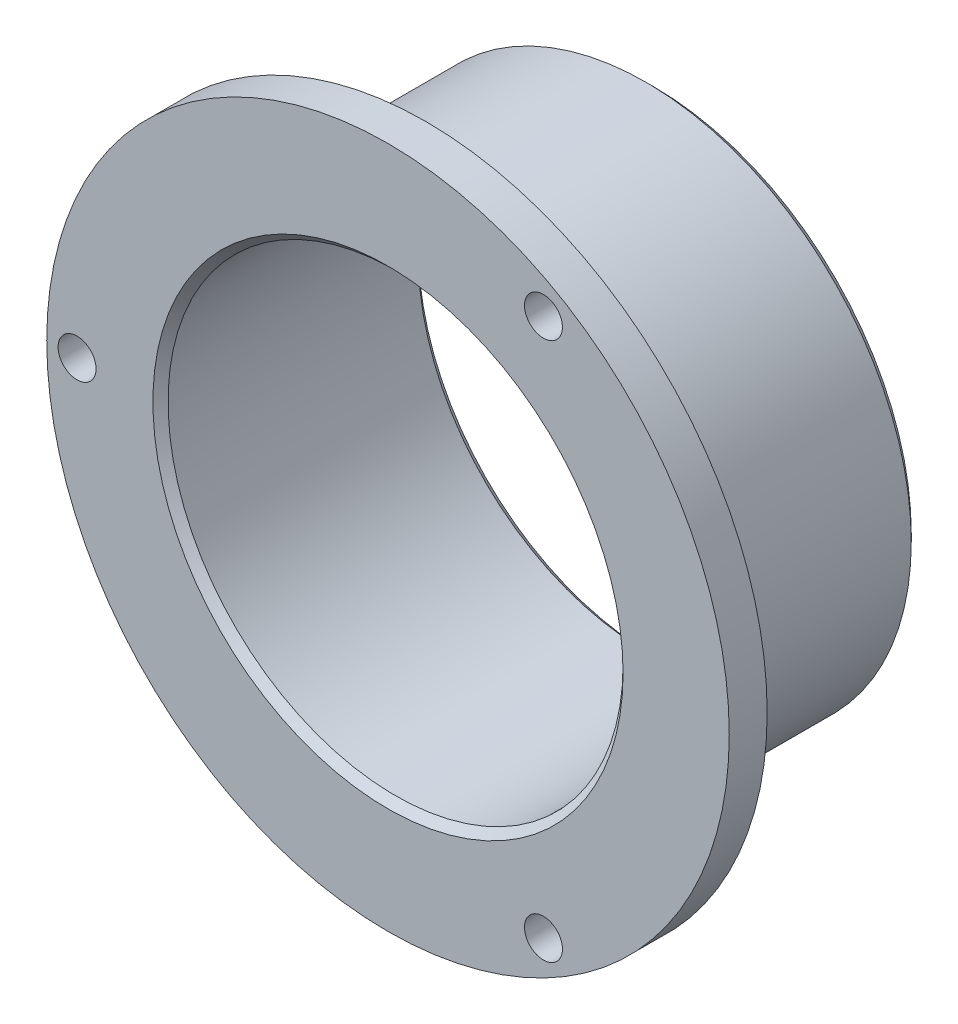
from build123d import *

# Parameters (mm, degrees)
SKETCH1_R           = 35
SKETCH1_R_2         = 30
BOSS_EXTRUDE1_DEPTH = 30
SKETCH2_R           = 45
SKETCH2_R_2         = 30
BOSS_EXTRUDE2_DEPTH = 5
SKETCH3_R           = 2.5
CUT_EXTRUDE1_DEPTH  = 50
CHAMFER1_SIZE       = 1


with BuildPart() as part:
    # Sketch1 → Boss-Extrude1 (new body)
    with BuildSketch(Plane.XY):
        Circle(SKETCH1_R)
        Circle(SKETCH1_R_2, mode=Mode.SUBTRACT)
    extrude(amount=BOSS_EXTRUDE1_DEPTH)

    # Sketch2 → Boss-Extrude2 (add)
    with BuildSketch(Plane.XY.offset(30)):
        Circle(SKETCH2_R)
        Circle(SKETCH2_R_2, mode=Mode.SUBTRACT)
    extrude(amount=BOSS_EXTRUDE2_DEPTH)

    # Sketch3 → Cut-Extrude1 (cut)
    with BuildSketch(Plane(origin=(0, 0, 30), x_dir=(-1, 0, 0), z_dir=(0, 0, -1))):
        with Locations((41, 0)):
            Circle(SKETCH3_R)
        with Locations((-20.5, -35.507041555)):
            Circle(SKETCH3_R)
        with Locations((-20.5, 35.507041555)):
            Circle(SKETCH3_R)
    extrude(amount=-CUT_EXTRUDE1_DEPTH, mode=Mode.SUBTRACT)

    # Chamfer1
    chamfer1_edges = [part.edges().sort_by_distance(p)[0] for p in [
        (-30, 0, 35),
        (-35, 0, 0),
        (-30, 0, 0),
    ]]
    chamfer(chamfer1_edges, length=CHAMFER1_SIZE)


solid = part.part
